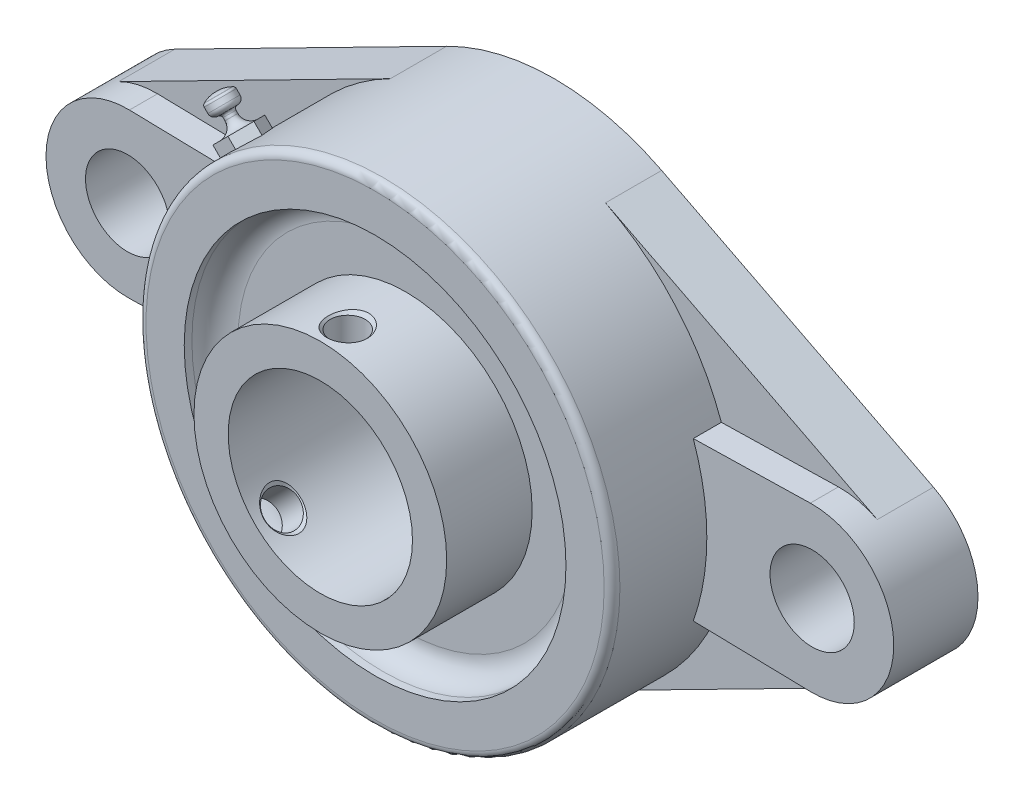
SolidWorks part; units mm, degrees
ref_plane "Front Plane" through (0, 0, 0) normal (0, 0, 1) x (1, 0, 0)
ref_plane "Top Plane" through (0, 0, 0) normal (0, 1, 0) x (1, 0, 0)
ref_plane "Right Plane" through (0, 0, 0) normal (1, 0, 0) x (0, 0, -1)
ref_plane "Plane1" through (0, 0, 0) normal (0.7071, 0.7071, 0) x (0, 0, -1)
sketch "Sketch1" plane through (0, 0, 0) normal (0.7071, 0.7071, 0) x (0, 0, -1)
  line L0 (-4.44, 53) -> (-4.2618, 53)
  line L1 (-2.2618, 52.4641) -> (-2.19, 52.4226)
  line L2 (-1.94, 51.9896) -> (-1.94, 51)
  line L3 (-3.44, 49.5) -> (-3.44, 49)
  line L4 (-1.44, 47) -> (0.56, 47)
  line L5 (0.56, 47) -> (0.56, 43)
  line L6 (0.56, 43) -> (-4.44, 43)
  line L7 (-4.44, 43) -> (-4.44, 53)
  line L8 (-4.44, 43) -> (-4.44, 53) construction
  arc A0 (-4.2618, 53) -> (-2.2618, 52.4641) centre (-4.2618, 49) cw
  arc A1 (-2.19, 52.4226) -> (-1.94, 51.9896) centre (-2.44, 51.9896) cw
  arc A2 (-1.94, 51) -> (-2.94, 50) centre (-2.94, 51) cw
  arc A3 (-2.94, 50) -> (-3.44, 49.5) centre (-2.94, 49.5) ccw
  arc A4 (-3.44, 49) -> (-1.44, 47) centre (-1.44, 49) ccw
revolve "Revolve1" add sketch "Sketch1" angle 360 about L8
ref_plane "Plane2" through (-30.4056, 30.4056, 0) normal (0.7071, -0.7071, 0) x (0, 0, -1)
sketch "Sketch2" plane through (-30.4056, 30.4056, 0) normal (0.7071, -0.7071, 0) x (0, 0, -1)
  line L0 (-9.6947, -5.2298) -> (0.5657, -5.2298)
  line L1 (0.5657, -5.2298) -> (0.5657, 5.0804)
  line L2 (0.5657, 5.0804) -> (-9.6947, 5.0804)
  line L3 (-9.6947, 5.0804) -> (-9.6947, -5.2298)
  line L4 (-7.94, 2.0207) -> (-7.94, -2.0207)
  line L5 (-7.94, -2.0207) -> (-4.44, -4.0415)
  line L6 (-4.44, -4.0415) -> (-0.94, -2.0207)
  line L7 (-0.94, -2.0207) -> (-0.94, 2.0207)
  line L8 (-0.94, 2.0207) -> (-4.44, 4.0415)
  line L9 (-4.44, 4.0415) -> (-7.94, 2.0207)
extrude "Cut-Extrude1" cut sketch "Sketch2" against normal blind 4
sketch "Sketch3" plane through (0, 0, 0) normal (1, 0, 0) x (0, 0, -1)
  line L0 (-22.2, 24) -> (-22.2, 17.5)
  line L1 (-22.2, 17.5) -> (20.7, 17.5)
  line L2 (20.7, 17.5) -> (20.7, 24)
  line L3 (20.7, 24) -> (19.5333, 24)
  line L4 (13.7, 29.8333) -> (13.7, 31.875)
  line L5 (18.075, 36.25) -> (22.2, 36.25)
  line L6 (22.2, 36.25) -> (22.2, 80.5)
  line L7 (22.2, 80.5) -> (6.2, 80.5)
  line L8 (6.2, 80.5) -> (6.2, 45)
  line L9 (6.2, 45) -> (-10.3, 45)
  line L10 (-11.8, 43.5) -> (-11.8, 36.25)
  line L11 (-11.8, 36.25) -> (-10.3417, 36.25)
  line L12 (-5.9667, 31.875) -> (-5.9667, 24)
  line L13 (-5.9667, 24) -> (-22.2, 24)
  line L14 (22.2, 0) -> (-22.2, 0) construction
  arc A0 (19.5333, 24) -> (13.7, 29.8333) centre (19.5333, 29.8333) cw
  arc A1 (13.7, 31.875) -> (18.075, 36.25) centre (18.075, 31.875) cw
  arc A2 (-10.3, 45) -> (-11.8, 43.5) centre (-10.3, 43.5) ccw
  arc A3 (-10.3417, 36.25) -> (-5.9667, 31.875) centre (-10.3417, 31.875) cw
revolve "Revolve2" add sketch "Sketch3" angle 360 about L14
sketch "Sketch4" plane through (0, 0, 0) normal (0, 0, 1) x (1, 0, 0)
  line L0 (-234, -180) -> (234, -180)
  line L1 (234, -180) -> (234, 180)
  line L2 (234, 180) -> (-234, 180)
  line L3 (-234, 180) -> (-234, -180)
  line L4 (-72.0346, -13.8117) -> (-20.4231, -40.0986)
  line L5 (20.4231, -40.0986) -> (72.0346, -13.8117)
  line L6 (72.0346, 13.8117) -> (20.4231, 40.0986)
  line L7 (-20.4231, 40.0986) -> (-72.0346, 13.8117)
  arc A0 (-72.0346, 13.8117) -> (-72.0346, -13.8117) centre (-65, 0) ccw
  arc A1 (-20.4231, -40.0986) -> (20.4231, -40.0986) centre (0, 0) ccw
  arc A2 (72.0346, -13.8117) -> (72.0346, 13.8117) centre (65, 0) ccw
  arc A3 (20.4231, 40.0986) -> (-20.4231, 40.0986) centre (0, 0) ccw
extrude "Cut-Extrude2" cut sketch "Sketch4" against normal blind 44.4
ref_plane "Plane3" through (0, 0, -6.2) normal (0, 0, 1) x (1, 0, 0)
sketch "Sketch5" plane through (0, 0, -6.2) normal (0, 0, 1) x (1, 0, 0)
  line L0 (-117, -90) -> (117, -90)
  line L1 (117, -90) -> (117, 90)
  line L2 (117, 90) -> (-117, 90)
  line L3 (-117, 90) -> (-117, -90)
  line L4 (-64.6541, -15.4961) -> (-42.4264, -15)
  line L5 (42.4264, -15) -> (64.6541, -15.4961)
  line L6 (64.6541, 15.4961) -> (42.4264, 15)
  line L7 (-42.4264, 15) -> (-64.6541, 15.4961)
  arc A0 (-64.6541, 15.4961) -> (-64.6541, -15.4961) centre (-65, 0) ccw
  arc A1 (-42.4264, -15) -> (42.4264, -15) centre (0, 0) ccw
  arc A2 (64.6541, -15.4961) -> (64.6541, 15.4961) centre (65, 0) ccw
  arc A3 (42.4264, 15) -> (-42.4264, 15) centre (0, 0) ccw
extrude "Cut-Extrude3" cut sketch "Sketch5" against normal blind 5.3333
sketch "Sketch6" plane through (0, 0, -6.2) normal (0, 0, 1) x (1, 0, 0)
  circle A0 centre (-65, 0) radius 8
sketch "Sketch7" plane through (0, 0, -6.2) normal (0, 0, 1) x (1, 0, 0)
  circle A0 centre (65, 0) radius 8
extrude "Cut-Extrude4" cut sketch "Sketch6" against normal blind 16
extrude "Cut-Extrude5" cut sketch "Sketch7" against normal blind 16
sketch "Sketch8" plane through (0, 0, 0) normal (1, 0, 0) x (0, 0, -1)
  line L0 (-17, 24) -> (-13, 24)
  line L1 (-13, 24) -> (-13.6765, 23.3235)
  line L2 (-13.6765, 23.3235) -> (-13.6765, 17.6765)
  line L3 (-13.6765, 17.6765) -> (-13, 17)
  line L4 (-13, 17) -> (-17, 17)
  line L5 (-17, 17) -> (-17, 24)
  line L6 (-17, 17) -> (-17, 24) construction
revolve "Cut-Revolve1" cut sketch "Sketch8" angle 360 about L6
cosmetic thread "Cosmetic Thread1" parameters "D1"=6.3235, "D2"=8
ref_plane "Plane4" through (0, 0, 0) normal (0.7071, -0.7071, 0) x (0, 0, -1)
sketch "Sketch9" plane through (0, 0, 0) normal (0.7071, -0.7071, 0) x (0, 0, -1)
  line L0 (-17, -17) -> (-13, -17)
  line L1 (-13, -17) -> (-13.6765, -17.6765)
  line L2 (-13.6765, -17.6765) -> (-13.6765, -23.3235)
  line L3 (-13.6765, -23.3235) -> (-13, -24)
  line L4 (-13, -24) -> (-17, -24)
  line L5 (-17, -24) -> (-17, -17)
  line L6 (-17, -24) -> (-17, -17) construction
revolve "Cut-Revolve2" cut sketch "Sketch9" angle 360 about L6
cosmetic thread "Cosmetic Thread2" parameters "D1"=6.2756, "D2"=8
ref_plane "Plane5" through (0, 0, 0) normal (0.7071, 0.7071, 0) x (-0.7071, 0.7071, 0)
